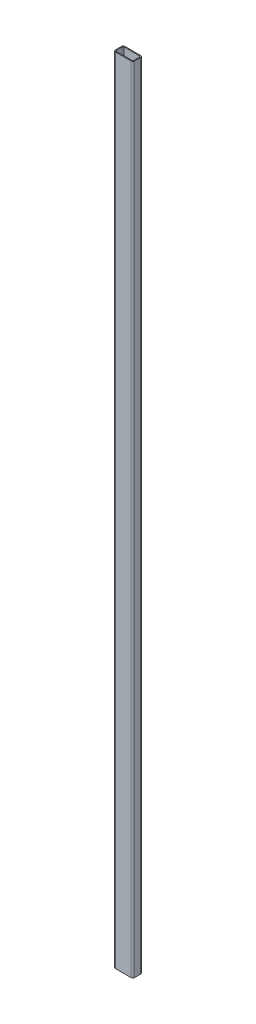
from build123d import *

# Parameters (mm, degrees)
EXTRUDE_1_DEPTH = 1650


with BuildPart() as part:
    # 草图1 → 凸台-拉伸1 (new body)
    with BuildSketch(Plane(origin=(0, 0, 0), x_dir=(1, 0, 0), z_dir=(0, 1, 0))):
        with BuildLine():
            Line((-16, -10), (16, -10))
            ThreePointArc((16, -10), (18.828427125, -8.828427125), (20, -6))
            Line((20, -6), (20, 6))
            ThreePointArc((20, 6), (18.828427125, 8.828427125), (16, 10))
            Line((16, 10), (-16, 10))
            ThreePointArc((-16, 10), (-18.828427125, 8.828427125), (-20, 6))
            Line((-20, 6), (-20, -6))
            ThreePointArc((-20, -6), (-18.828427125, -8.828427125), (-16, -10))
        make_face()
        with BuildLine():
            Line((-16, -8), (16, -8))
            ThreePointArc((16, -8), (17.414213562, -7.414213562), (18, -6))
            Line((18, -6), (18, 6))
            ThreePointArc((18, 6), (17.414213562, 7.414213562), (16, 8))
            Line((16, 8), (-16, 8))
            ThreePointArc((-16, 8), (-17.414213562, 7.414213562), (-18, 6))
            Line((-18, 6), (-18, -6))
            ThreePointArc((-18, -6), (-17.414213562, -7.414213562), (-16, -8))
        make_face(mode=Mode.SUBTRACT)
    extrude(amount=EXTRUDE_1_DEPTH)


solid = part.part
